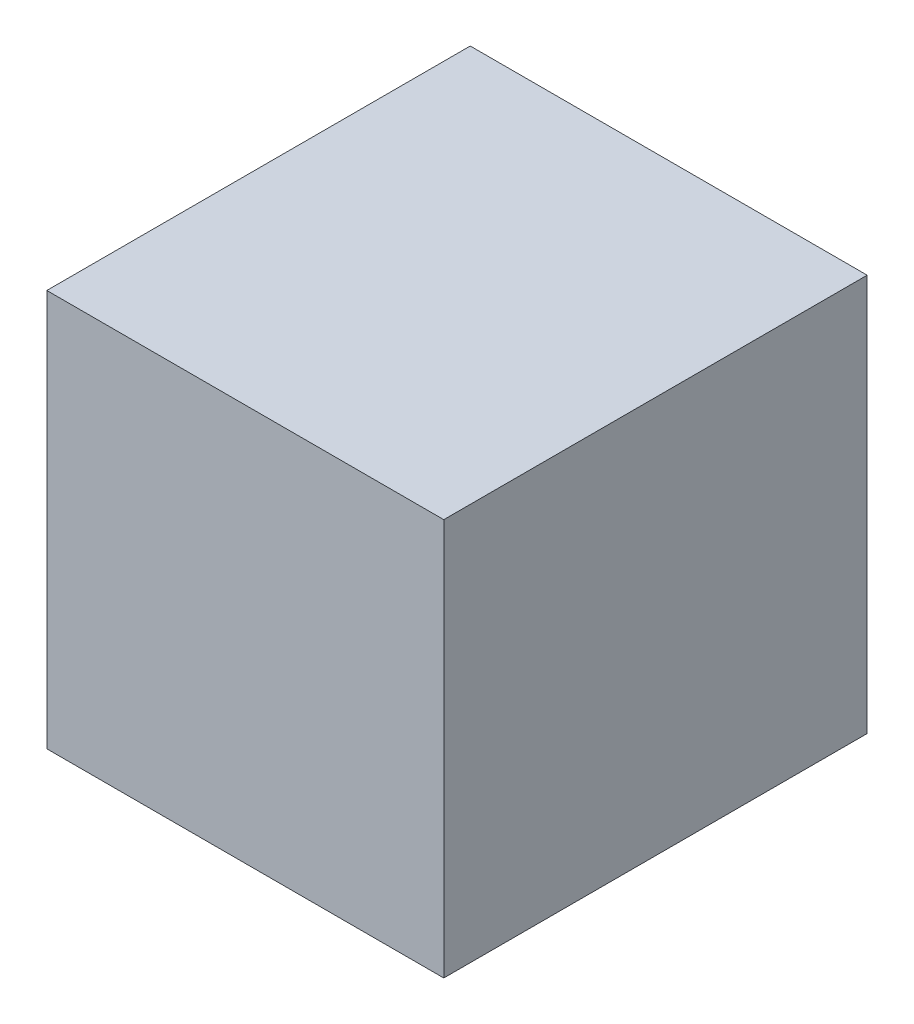
SolidWorks part; units mm, degrees
ref_plane "前视基准面" through (0, 0, 0) normal (0, 0, 1) x (1, 0, 0)
ref_plane "上视基准面" through (0, 0, 0) normal (0, 1, 0) x (1, 0, 0)
ref_plane "右视基准面" through (0, 0, 0) normal (1, 0, 0) x (0, 0, -1)
sketch "草图1" plane through (0, 0, 0) normal (0, 0, 1) x (1, 0, 0)
  line L1 (-37.5, 37.5) -> (37.5, 37.5)
  line L2 (-37.5, 37.5) -> (-37.5, -37.5)
  line L3 (-37.5, -37.5) -> (37.5, -37.5)
  line L4 (37.5, 37.5) -> (37.5, -37.5)
  line L5 (-37.5, 37.5) -> (37.5, -37.5) construction
  line L6 (-37.5, -37.5) -> (37.5, 37.5) construction
  point P0 (0, 0)
  dimension "D1" = 75
  dimension "D2" = 75
extrude "凸台-拉伸1" add sketch "草图1" along normal blind 80
hole_wizard "M6 螺纹孔2" positions "草图5" profile "草图4" tap size "M6" standard "ISO"
sketch "草图5" plane through (0, 0, 0) normal (0, 0, -1) x (-1, 0, 0)
  line L0 (-37.5, -37.5) -> (-37.5, 37.5) construction
  line L1 (-37.5, 37.5) -> (37.5, 37.5) construction
  line L2 (50.3247, 0) -> (-66.3282, 0) construction
  point P0 (-31.5, 31)
  point P2 (-20.5, 31)
  point P4 (20.5, 31)
  point P14 (20.5, -31)
  point P15 (-20.5, -31)
  point P16 (-31.5, -31)
  dimension "D1" = 6
  dimension "D2" = 6.5
  dimension "D3" = 11
  dimension "D4" = 41
sketch "草图4" plane through (31.5, 31, 0) normal (1, 0, 0) x (0, 1, 0)
  line L0 (0, 0) -> (0, 16.5022)
  line L1 (0, 16.5022) -> (2.5, 15)
  line L2 (2.5, 15) -> (2.5, 0)
  line L5 (2.5, 0) -> (0, 0)
  line L10 (0, 16.5022) -> (-2.5, 15) construction
  line L11 (0, -6.35) -> (0, 107.95) construction
  dimension "螺纹孔钻头直径" = 5
  dimension "螺纹孔钻头深度" = 15
  dimension "导头角度" = 118
cosmetic thread "孔螺蚊线7"
cosmetic thread "孔螺蚊线8"
cosmetic thread "孔螺蚊线9"
cosmetic thread "孔螺蚊线10"
cosmetic thread "孔螺蚊线11"
cosmetic thread "孔螺蚊线12"
